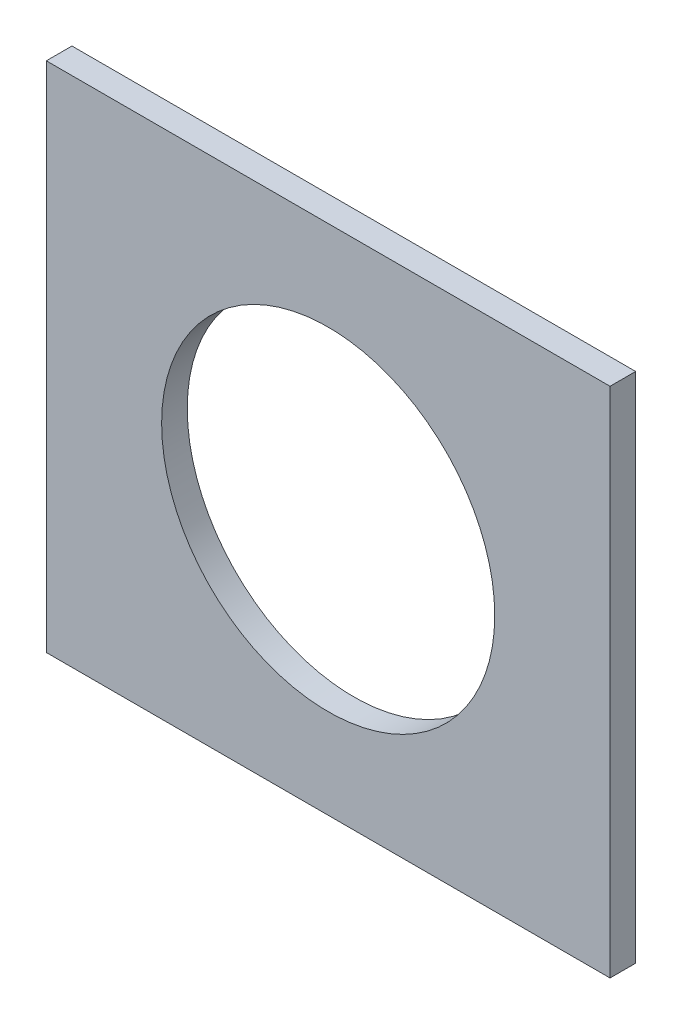
from build123d import *

# Parameters (mm, degrees)
SKETCH_1_W          = 110
SKETCH_1_H          = 100
EXTRUDE_1_DEPTH     = 5
CUT_EXTRUDE_1_DEPTH = 5
SKETCH_3_W          = 5
SKETCH_3_H          = 100
EXTRUDE_2_DEPTH     = 50
SKETCH_4_W          = 5
SKETCH_4_H          = 100
EXTRUDE_3_DEPTH     = 50
SKETCH_5_W          = 5
SKETCH_5_H          = 100
CUT_EXTRUDE_2_DEPTH = 50
SKETCH_7_W          = 5
SKETCH_7_H          = 100
CUT_EXTRUDE_3_DEPTH = 50


with BuildPart() as part:
    # 草图1 → 凸台-拉伸1 (new body)
    with BuildSketch(Plane.XY):
        with Locations((55, 50)):
            Rectangle(SKETCH_1_W, SKETCH_1_H)
    extrude(amount=EXTRUDE_1_DEPTH)

    # 草图2 → 切除-拉伸1 (cut)
    with BuildSketch(Plane.XY.offset(5)):
        with BuildLine():
            Line((55, 50), (79.048052385, 71.861865805))
            ThreePointArc((79.048052385, 71.861865805), (68.147991507, 79.72171461), (55, 82.5))
            Line((55, 82.5), (55, 50))
        make_face()
        with BuildLine():
            Line((30.951947615, 28.138134195), (55, 50))
            Line((55, 50), (55, 82.5))
            ThreePointArc((55, 82.5), (25.27828539, 63.147991507), (30.951947615, 28.138134195))
        make_face()
        with BuildLine():
            ThreePointArc((87.5, 50), (85.313459903, 61.719391995), (79.048052385, 71.861865805))
            Line((79.048052385, 71.861865805), (55, 50))
            Line((55, 50), (30.951947615, 28.138134195))
            ThreePointArc((30.951947615, 28.138134195), (66.719391995, 19.686540097), (87.5, 50))
        make_face()
    extrude(amount=-CUT_EXTRUDE_1_DEPTH, mode=Mode.SUBTRACT)

    # 草图3 → 凸台-拉伸2 (add)
    with BuildSketch(Plane(origin=(110, 0, 0), x_dir=(0, 0, -1), z_dir=(1, 0, 0))):
        with Locations((-2.5, 50)):
            Rectangle(SKETCH_3_W, SKETCH_3_H)
    extrude(amount=EXTRUDE_2_DEPTH)

    # 草图4 → 凸台-拉伸3 (add)
    with BuildSketch(Plane.ZY):
        with Locations((2.5, 50)):
            Rectangle(SKETCH_4_W, SKETCH_4_H)
    extrude(amount=EXTRUDE_3_DEPTH)

    # 草图5 → 切除-拉伸2 (cut)
    with BuildSketch(Plane(origin=(160, 0, 0), x_dir=(0, 0, -1), z_dir=(1, 0, 0))):
        with Locations((-2.5, 50)):
            Rectangle(SKETCH_5_W, SKETCH_5_H)
    extrude(amount=-CUT_EXTRUDE_2_DEPTH, mode=Mode.SUBTRACT)

    # 草图7 → 切除-拉伸3 (cut)
    with BuildSketch(Plane.ZY.offset(50)):
        with Locations((2.5, 50)):
            Rectangle(SKETCH_7_W, SKETCH_7_H)
    extrude(amount=-CUT_EXTRUDE_3_DEPTH, mode=Mode.SUBTRACT)


solid = part.part
